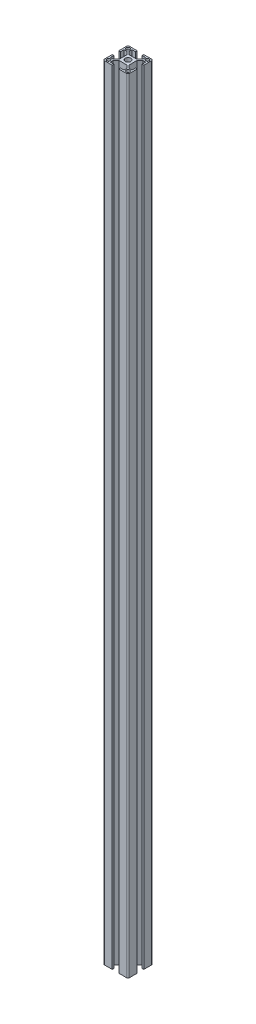
from build123d import *

# Parameters (mm, degrees)
SKETCH_1_R      = 2.1
SKETCH_1_R_2    = 3.4
EXTRUDE_1_DEPTH = 940


with BuildPart() as part:
    # 草图1 → 拉伸1 (new body)
    with BuildSketch(Plane(origin=(0, 0, 0), x_dir=(1, 0, 0), z_dir=(0, 1, 0))):
        with BuildLine():
            Line((6.75, -28), (11, -28))
            Line((11, -28), (11, -30))
            Line((11, -30), (2, -30))
            ThreePointArc((2, -30), (0.585786438, -29.414213562), (0, -28))
            Line((0, -28), (0, -19))
            Line((0, -19), (2, -19))
            Line((2, -19), (2, -23.25))
            Line((2, -23.25), (5.335785999, -23.25))
            Line((5.335785999, -23.25), (9, -19.585785999))
            Line((9, -19.585785999), (9, -10.414214001))
            Line((9, -10.414214001), (5.335785999, -6.75))
            Line((5.335785999, -6.75), (2, -6.75))
            Line((2, -6.75), (2, -11))
            Line((2, -11), (0, -11))
            Line((0, -11), (0, -2))
            ThreePointArc((0, -2), (0.585786438, -0.585786438), (2, 0))
            Line((2, 0), (11, 0))
            Line((11, 0), (11, -2))
            Line((11, -2), (6.75, -2))
            Line((6.75, -2), (6.75, -5.335785999))
            Line((6.75, -5.335785999), (10.414214001, -9))
            Line((10.414214001, -9), (19.585785999, -9))
            Line((19.585785999, -9), (23.25, -5.335785999))
            Line((23.25, -5.335785999), (23.25, -2))
            Line((23.25, -2), (19, -2))
            Line((19, -2), (19, 0))
            Line((19, 0), (28, 0))
            ThreePointArc((28, 0), (29.414213562, -0.585786438), (30, -2))
            Line((30, -2), (30, -11))
            Line((30, -11), (28, -11))
            Line((28, -11), (28, -6.75))
            Line((28, -6.75), (24.664214001, -6.75))
            Line((24.664214001, -6.75), (21, -10.414214001))
            Line((21, -10.414214001), (21, -19.585785999))
            Line((21, -19.585785999), (24.664214001, -23.25))
            Line((24.664214001, -23.25), (28, -23.25))
            Line((28, -23.25), (28, -19))
            Line((28, -19), (30, -19))
            Line((30, -19), (30, -28))
            ThreePointArc((30, -28), (29.414213562, -29.414213562), (28, -30))
            Line((28, -30), (19, -30))
            Line((19, -30), (19, -28))
            Line((19, -28), (23.25, -28))
            Line((23.25, -28), (23.25, -24.664214001))
            Line((23.25, -24.664214001), (19.585785999, -21))
            Line((19.585785999, -21), (10.414214001, -21))
            Line((10.414214001, -21), (6.75, -24.664214001))
            Line((6.75, -24.664214001), (6.75, -28))
        make_face()
        with Locations(Location((3.375, -26.625, 0), (0, 0, 90))):
            Circle(SKETCH_1_R, mode=Mode.SUBTRACT)
        with Locations(Location((26.625, -26.625, 0), (0, 0, 90))):
            Circle(SKETCH_1_R, mode=Mode.SUBTRACT)
        with Locations(Location((15, -15, 0), (0, 0, 90))):
            Circle(SKETCH_1_R_2, mode=Mode.SUBTRACT)
        with Locations(Location((3.375, -3.375, 0), (0, 0, 90))):
            Circle(SKETCH_1_R, mode=Mode.SUBTRACT)
        with Locations(Location((26.625, -3.375, 0), (0, 0, 90))):
            Circle(SKETCH_1_R, mode=Mode.SUBTRACT)
    extrude(amount=EXTRUDE_1_DEPTH)


solid = part.part
